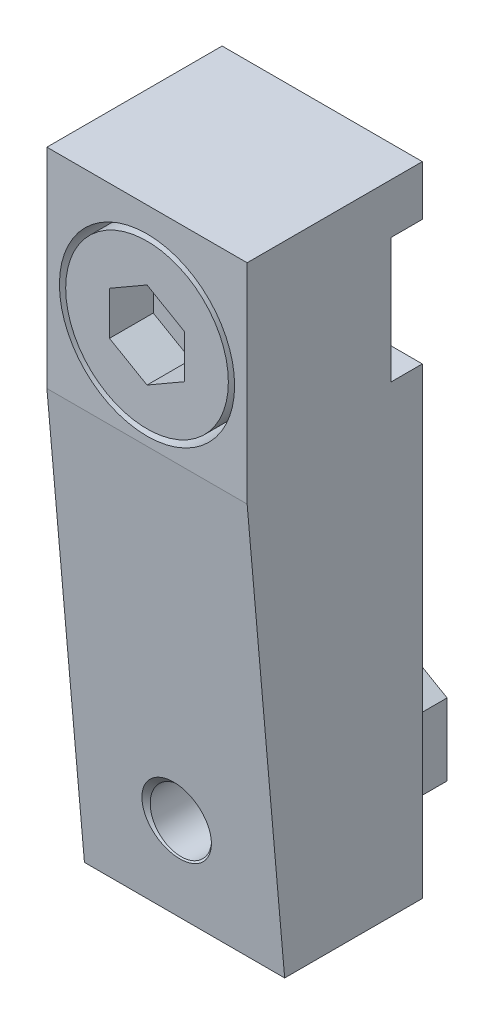
from build123d import *

# Parameters (mm, degrees)
EXTRUDE_1_DEPTH      = 8
EXTRUDE_1_DEPTH_BACK = 8
SKETCH_2_W           = 16
SKETCH_2_H           = 10
CUT_EXTRUDE_1_DEPTH  = 2.5
SKETCH_3_W           = 5
SKETCH_3_H           = 5.75
SKETCH_4_R           = 11.5
CUT_EXTRUDE_2_DEPTH  = 5
SKETCH_6_R           = 7
SKETCH_6_R_2         = 6.5
CUT_EXTRUDE_3_DEPTH  = 7
CUT_EXTRUDE_4_DEPTH  = 3.5


with BuildPart() as part:
    # 草图1 → 凸台-拉伸1 (new, two sides: drawn at the far end of the back side and taken through both)
    with BuildSketch(Plane(origin=(0, 0, 0), x_dir=(0, 0, -1), z_dir=(1, 0, 0)).offset(-EXTRUDE_1_DEPTH_BACK)):
        Polygon((-11.5, 9), (-11.5, -7.7), (-8.5, -42), (2.5, -42), (2.5, 9), align=None)
    extrude(amount=EXTRUDE_1_DEPTH + EXTRUDE_1_DEPTH_BACK)

    # 草图2 → 切除-拉伸1 (cut)
    with BuildSketch(Plane.XY):
        Rectangle(SKETCH_2_W, SKETCH_2_H)
    extrude(amount=-CUT_EXTRUDE_1_DEPTH, mode=Mode.SUBTRACT)

    # 草图3 → 旋转1 (revolve)
    with BuildSketch(Plane(origin=(0, 0, 0), x_dir=(0, 0, -1), z_dir=(1, 0, 0)), mode=Mode.PRIVATE) as revolve_1_sk:
        with Locations((5, -32.125)):
            Rectangle(SKETCH_3_W, SKETCH_3_H)
    revolve(revolve_1_sk.sketch.rotate(Axis((0, -35, -7.5), (0, 0, 1)), 270), axis=Axis((0, -35, -7.5), (0, 0, 1)))

    # 草图4 → 切除-拉伸2 (cut)
    with BuildSketch(Plane(origin=(0, 0, -7.5), x_dir=(-1, 0, 0), z_dir=(0, 0, -1))):
        with Locations((0, -35)):
            Circle(SKETCH_4_R)
        Polygon((0, -40.75), (4.979646072, -37.875), (4.979646072, -32.125), (0, -29.25), (-4.979646072, -32.125), (-4.979646072, -37.875), align=None, mode=Mode.SUBTRACT)
    extrude(amount=-CUT_EXTRUDE_2_DEPTH, mode=Mode.SUBTRACT)

    # 草图5 → 切除-旋转1 (revolve, cut)
    with BuildSketch(Plane(origin=(0, 0, 0), x_dir=(0, 0, -1), z_dir=(1, 0, 0)), mode=Mode.PRIVATE) as cut_revolve_1_sk:
        Polygon((-9.112244898, -35), (-9.374635569, -32), (-8.785774052, -32.5415), (6.9585, -32.5415), (7.5, -32), (7.5, -35), align=None)
    revolve(cut_revolve_1_sk.sketch.rotate(Axis((0, -35, -7.5), (0, 0, 1)), 270), axis=Axis((0, -35, -7.5), (0, 0, 1)), mode=Mode.SUBTRACT)

    # 草图6 → 切除-拉伸3 (cut)
    with BuildSketch(Plane.XY.offset(11.5)):
        Circle(SKETCH_6_R)
        Circle(SKETCH_6_R_2, mode=Mode.SUBTRACT)
    extrude(amount=-CUT_EXTRUDE_3_DEPTH, mode=Mode.SUBTRACT)

    # 草图7 → 切除-拉伸4 (cut)
    with BuildSketch(Plane.XY.offset(11.5)):
        Polygon((-3, 1.732050808), (-3, -1.732050808), (0, -3.464101615), (3, -1.732050808), (3, 1.732050808), (0, 3.464101615), align=None)
    extrude(amount=-CUT_EXTRUDE_4_DEPTH, mode=Mode.SUBTRACT)


solid = part.part
